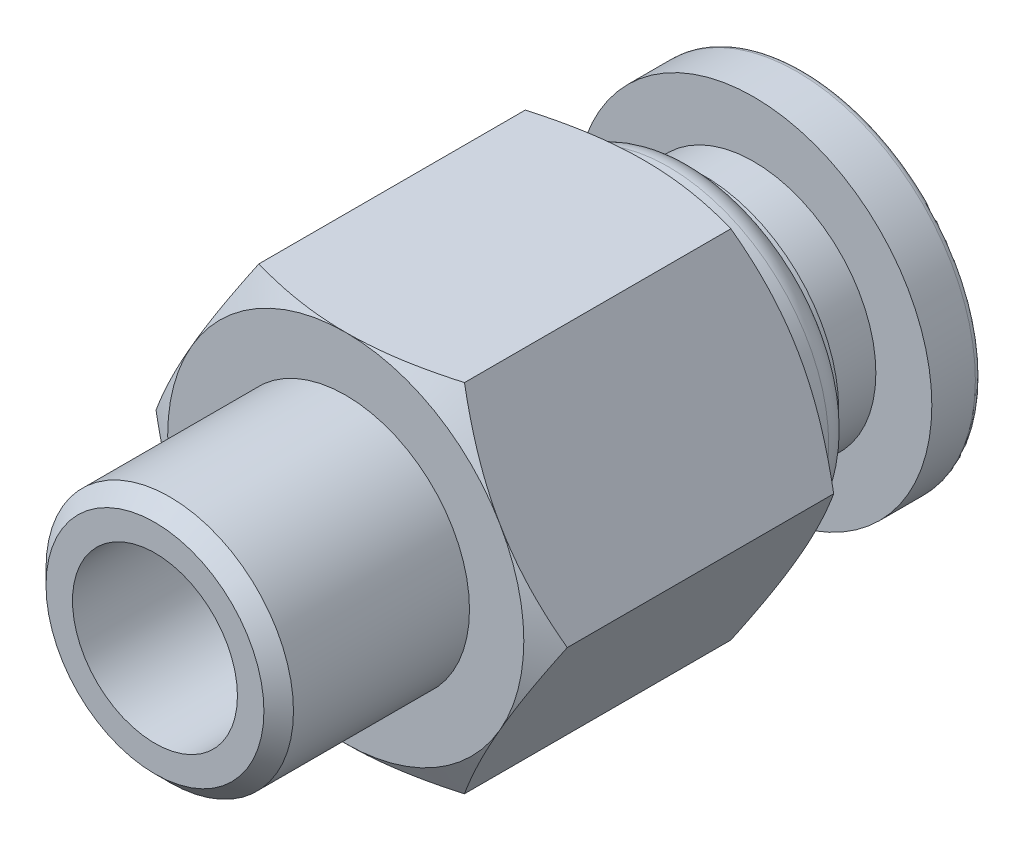
from build123d import *

# Parameters (mm, degrees)
SKETCH_2_R          = 14
CUT_EXTRUDE_1_DEPTH = 25.5


with BuildPart() as part:
    # 草图1 → 旋转1 (revolve)
    with BuildSketch(Plane(origin=(0, 0, 0), x_dir=(0, 0, -1), z_dir=(1, 0, 0)), mode=Mode.PRIVATE) as revolve_1_sk:
        with BuildLine():
            Line((-25.5, 3.242666667), (-17, 3.242666667))
            Line((-17, 3.242666667), (-17, 4))
            Line((-17, 4), (0, 4))
            Line((0, 4), (0, 6.75))
            ThreePointArc((0, 6.75), (-0.073223305, 6.926776695), (-0.25, 7))
            Line((-0.25, 7), (-1.961538462, 7))
            Line((-1.961538462, 7), (-1.961538462, 4.8))
            Line((-1.961538462, 4.8), (-3.923076923, 4.8))
            Line((-3.923076923, 4.8), (-3.923076923, 5.3))
            Line((-3.923076923, 5.3), (-4.315384615, 5.3))
            ThreePointArc((-4.315384615, 5.3), (-4.608277834, 6.007106781), (-5.315384615, 6.3))
            Line((-5.315384615, 6.3), (-6.276923077, 6.3))
            Line((-6.276923077, 6.3), (-6.276923077, 7))
            Line((-6.276923077, 7), (-6.902137859, 8.082903769))
            Line((-6.902137859, 8.082903769), (-17.374785218, 8.082903769))
            Line((-17.374785218, 8.082903769), (-18, 7))
            Line((-18, 7), (-18, 4.864))
            Line((-18, 4.864), (-24.919, 4.864))
            Line((-24.919, 4.864), (-25.5, 4.283))
            Line((-25.5, 4.283), (-25.5, 3.242666667))
        make_face()
    revolve(revolve_1_sk.sketch.rotate(Axis((0, 0, 0), (0, 0, 1)), 270), axis=Axis((0, 0, 0), (0, 0, 1)))

    # 草图2 → 切除-拉伸1 (cut)
    with BuildSketch(Plane(origin=(0, 0, 6.276923077), x_dir=(-1, 0, 0), z_dir=(0, 0, -1))):
        Circle(SKETCH_2_R)
        Polygon((-4.041451884, -7), (4.041451884, -7), (8.082903769, 0), (4.041451884, 7), (-4.041451884, 7), (-8.082903769, 0), align=None, mode=Mode.SUBTRACT)
    extrude(amount=-CUT_EXTRUDE_1_DEPTH, mode=Mode.SUBTRACT)


solid = part.part
